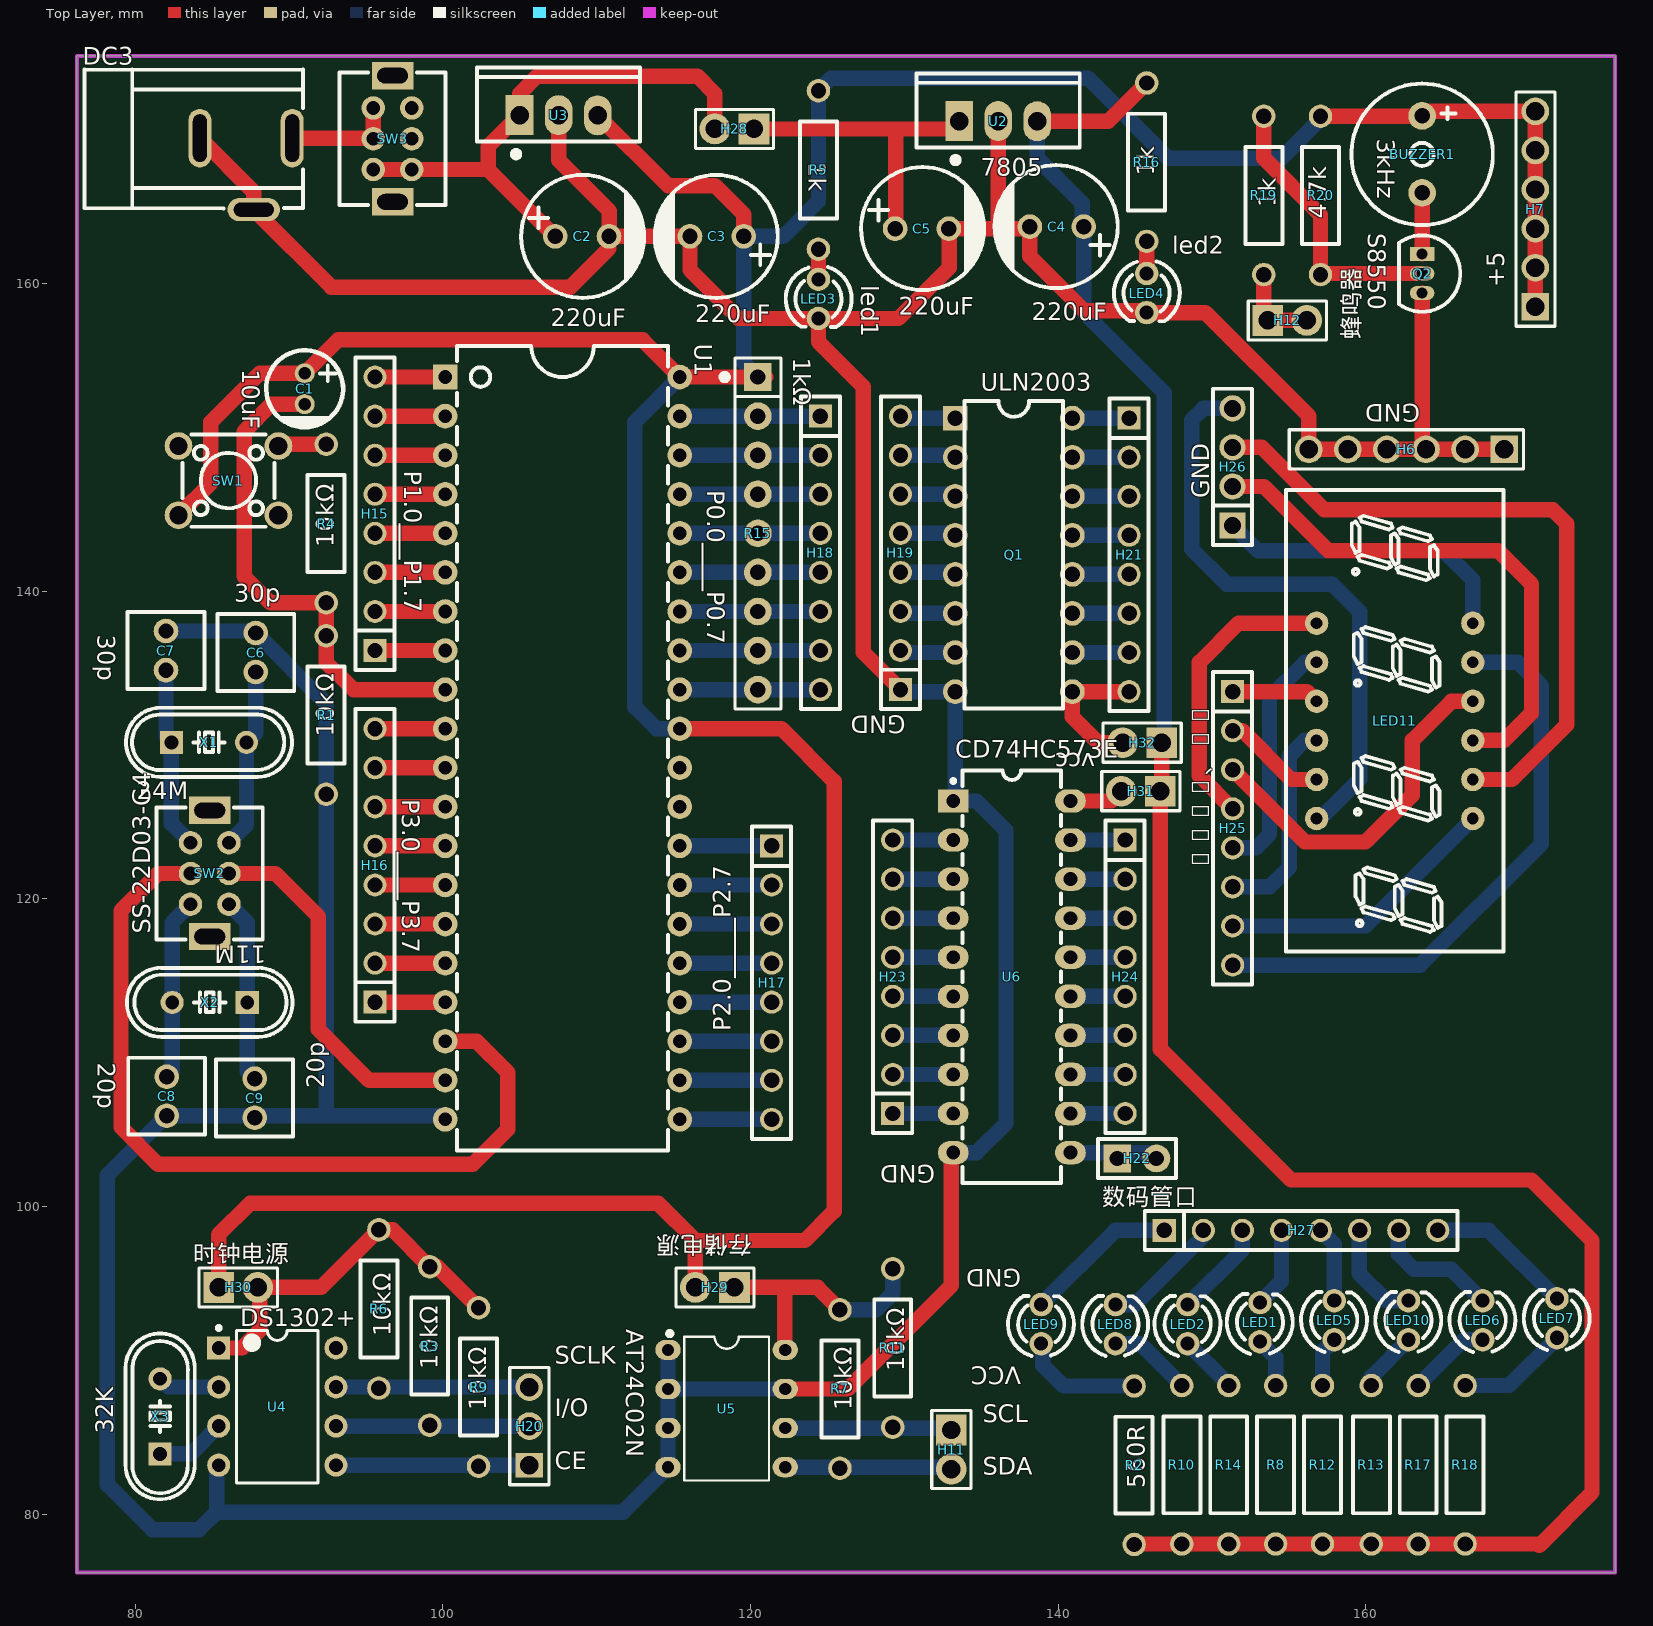
[diagram p0: Top Layer view]
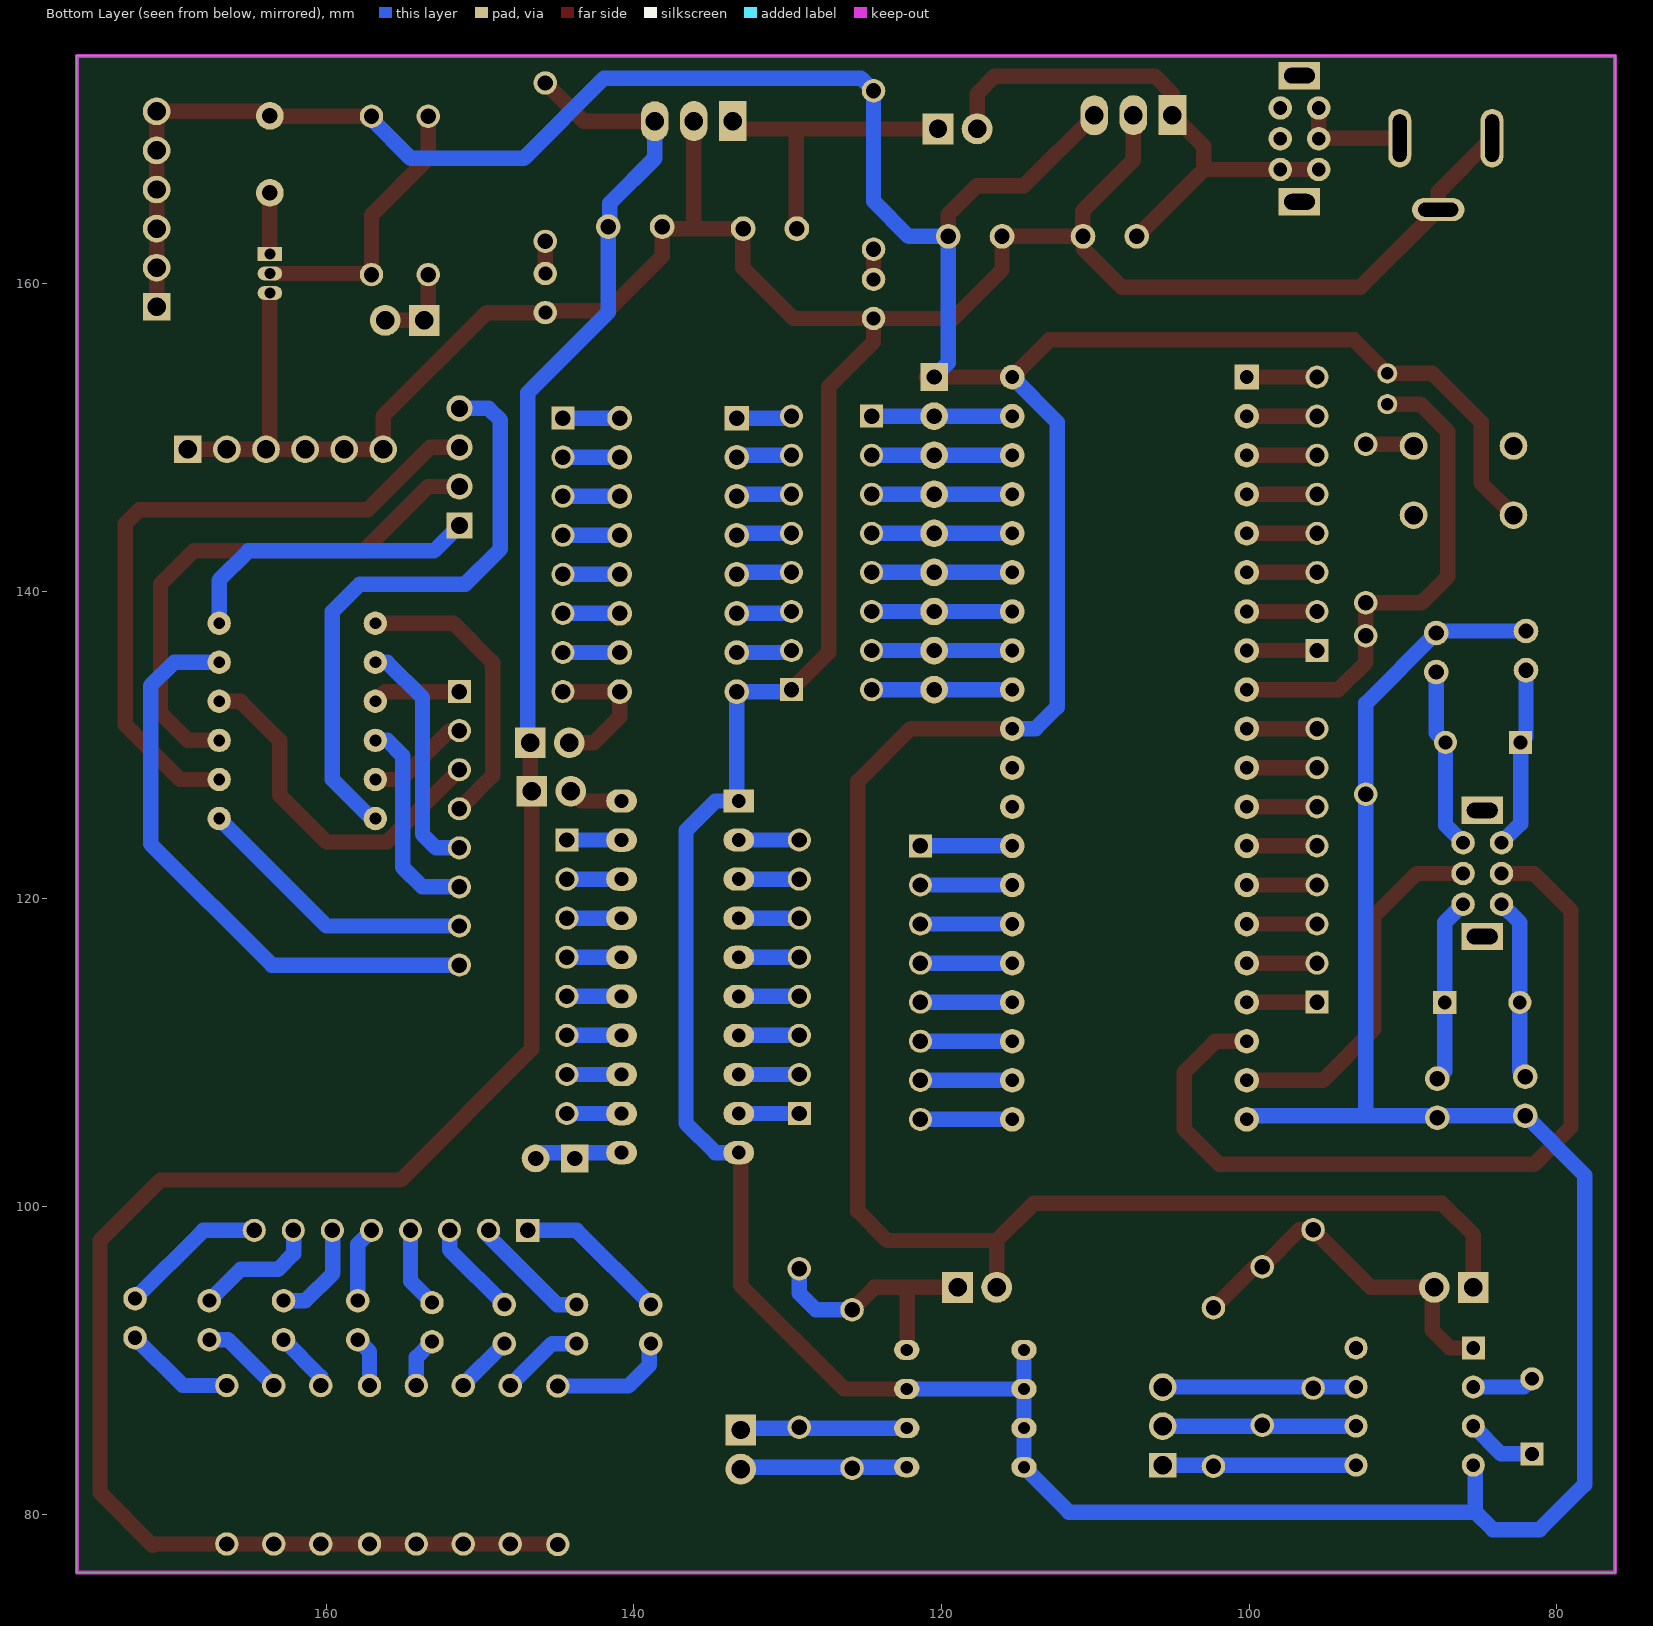
[diagram p1: Bottom Layer view, seen from below]
# Altium PCB MISC49922.pcbdoc
Units mm, origin at the board's own origin, x right, y up, seen from the top; angles counter-clockwise.
Board outline 100 x 98.6 mm, 2 copper layers (Top Layer, Bottom Layer), stack 1.58 mm thick; 78 components, 121 nets, 344 pads, 0 vias.

## Layer stack, top to bottom
Top Solder Mask Layer: solder mask 0.01, Dk 3.3
Top Layer: signal copper 0.035
Dielectric1: surface 1.51, FR4, Dk 4.5
Bottom Layer: signal copper 0.035
Bottom Solder Mask Layer: solder mask 0.01, Dk 3.3

## Board outline
76.2,174.803 76.2,76.2 176.2,76.2 176.2,174.803

## Design rules (kind name [scope] priority, off if disabled: settings)
BoardOutlineClearance copperThickness2oz_1 [All] p2 off: genericclearance=0.203 ignorepadtopadclearanceinfootprint=FALSE except(0: Arc-SplitContinuation Track-SplitContinuation SMDPad-SplitContinuation THPad-SplitContinuation Via-SplitContinuation Fill-SplitContinuation Region-SplitContinuation Poly-SplitContinuation Text-SplitContinuation Hole-SplitContinuation; 0.152: SMDPad-CutoutEdge THPad-CutoutEdge Via-CutoutEdge Fill-CutoutEdge Region-CutoutEdge Text-CutoutEdge Hole-CutoutEdge; 0.254: Poly-OutlineEdge Poly-CutoutEdge; 0.3: Arc-OutlineEdge Track-OutlineEdge SMDPad-OutlineEdge THPad-OutlineEdge Via-OutlineEdge Fill-OutlineEdge Region-OutlineEdge Text-OutlineEdge Hole-OutlineEdge Arc-CutoutEdge Track-CutoutEdge)
BoardOutlineClearance Plane_innerPlane_1 [All] p4 off: genericclearance=0.102 ignorepadtopadclearanceinfootprint=FALSE except(0: Arc-SplitContinuation Track-SplitContinuation SMDPad-SplitContinuation THPad-SplitContinuation Via-SplitContinuation Fill-SplitContinuation Region-SplitContinuation Poly-SplitContinuation Text-SplitContinuation Hole-SplitContinuation; 0.152: SMDPad-CutoutEdge THPad-CutoutEdge Via-CutoutEdge Fill-CutoutEdge Region-CutoutEdge Text-CutoutEdge Hole-CutoutEdge; 0.254: Poly-OutlineEdge Poly-CutoutEdge; 0.3: Arc-OutlineEdge Track-OutlineEdge SMDPad-OutlineEdge THPad-OutlineEdge Via-OutlineEdge Fill-OutlineEdge Region-OutlineEdge Text-OutlineEdge Hole-OutlineEdge Arc-CutoutEdge Track-CutoutEdge)
BoardOutlineClearance Copper_copperRegion_1 [All] p6 off: genericclearance=0.102 ignorepadtopadclearanceinfootprint=FALSE except(0: Arc-SplitContinuation Track-SplitContinuation SMDPad-SplitContinuation THPad-SplitContinuation Via-SplitContinuation Fill-SplitContinuation Region-SplitContinuation Poly-SplitContinuation Text-SplitContinuation Hole-SplitContinuation; 0.152: SMDPad-CutoutEdge THPad-CutoutEdge Via-CutoutEdge Fill-CutoutEdge Region-CutoutEdge Text-CutoutEdge Hole-CutoutEdge; 0.254: Poly-OutlineEdge Poly-CutoutEdge; 0.3: Arc-OutlineEdge Track-OutlineEdge SMDPad-OutlineEdge THPad-OutlineEdge Via-OutlineEdge Fill-OutlineEdge Region-OutlineEdge Text-OutlineEdge Hole-OutlineEdge Arc-CutoutEdge Track-CutoutEdge)
BoardOutlineClearance copperThickness1oz_1 [All] p8: genericclearance=0.102 ignorepadtopadclearanceinfootprint=FALSE except(0: Arc-SplitContinuation Track-SplitContinuation SMDPad-SplitContinuation THPad-SplitContinuation Via-SplitContinuation Fill-SplitContinuation Region-SplitContinuation Poly-SplitContinuation Text-SplitContinuation Hole-SplitContinuation; 0.152: SMDPad-CutoutEdge THPad-CutoutEdge Via-CutoutEdge Fill-CutoutEdge Region-CutoutEdge Text-CutoutEdge Hole-CutoutEdge; 0.254: Poly-OutlineEdge Poly-CutoutEdge; 0.3: Arc-OutlineEdge Track-OutlineEdge SMDPad-OutlineEdge THPad-OutlineEdge Via-OutlineEdge Fill-OutlineEdge Region-OutlineEdge Text-OutlineEdge Hole-OutlineEdge Arc-CutoutEdge Track-CutoutEdge)
Clearance copperThickness2oz [All] p1 off: gap=0.203 ignorepadtopadclearanceinfootprint=FALSE except(0.152: SMDPad-Track SMDPad-SMDPad THPad-Track SMDPad-THPad THPad-THPad Track-Via SMDPad-Via THPad-Via Via-Via Fill-Track Region-Track Fill-SMDPad Region-SMDPad Fill-THPad Region-THPad Fill-Via Region-Via Fill-Fill Fill-Region Region-Region Arc-Track Arc-SMDPad Arc-THPad Arc-Via Fill-Arc Region-Arc Arc-Arc Text-Track SMDPad-Text Text-THPad Text-Via Fill-Text Region-Text Arc-Text Text-Text Hole-Track Hole-SMDPad Hole-THPad Hole-Via Fill-Hole Region-Hole Hole-Arc Hole-Text; 0.254: Poly-Track Poly-SMDPad Poly-THPad Poly-Via Poly-Fill Poly-Region Poly-Poly Poly-Arc Poly-Text Poly-Hole)
Clearance Plane_innerPlane [All] p3 off: gap=0.102 ignorepadtopadclearanceinfootprint=FALSE except(0.152: SMDPad-Track SMDPad-SMDPad THPad-Track SMDPad-THPad THPad-THPad Track-Via SMDPad-Via THPad-Via Via-Via Fill-Track Region-Track Fill-SMDPad Region-SMDPad Fill-THPad Region-THPad Fill-Via Region-Via Fill-Fill Fill-Region Region-Region Arc-Track Arc-SMDPad Arc-THPad Arc-Via Fill-Arc Region-Arc Arc-Arc Text-Track SMDPad-Text Text-THPad Text-Via Fill-Text Region-Text Arc-Text Text-Text Hole-Track Hole-SMDPad Hole-THPad Hole-Via Fill-Hole Region-Hole Hole-Arc Hole-Text; 0.254: Poly-Track Poly-SMDPad Poly-THPad Poly-Via Poly-Fill Poly-Region Poly-Poly Poly-Arc Poly-Text Poly-Hole)
Clearance Copper_copperRegion [All] p5 off: gap=0.102 ignorepadtopadclearanceinfootprint=FALSE except(0.152: SMDPad-Track SMDPad-SMDPad THPad-Track SMDPad-THPad THPad-THPad Track-Via SMDPad-Via THPad-Via Via-Via Fill-Track Region-Track Fill-SMDPad Region-SMDPad Fill-THPad Region-THPad Fill-Via Region-Via Fill-Fill Fill-Region Region-Region Arc-Track Arc-SMDPad Arc-THPad Arc-Via Fill-Arc Region-Arc Arc-Arc Text-Track SMDPad-Text Text-THPad Text-Via Fill-Text Region-Text Arc-Text Text-Text Hole-Track Hole-SMDPad Hole-THPad Hole-Via Fill-Hole Region-Hole Hole-Arc Hole-Text; 0.254: Poly-Track Poly-SMDPad Poly-THPad Poly-Via Poly-Fill Poly-Region Poly-Poly Poly-Arc Poly-Text Poly-Hole)
Clearance copperThickness1oz [All] p7: gap=0.102 ignorepadtopadclearanceinfootprint=FALSE except(0.152: SMDPad-Track SMDPad-SMDPad THPad-Track SMDPad-THPad THPad-THPad Track-Via SMDPad-Via THPad-Via Via-Via Fill-Track Region-Track Fill-SMDPad Region-SMDPad Fill-THPad Region-THPad Fill-Via Region-Via Fill-Fill Fill-Region Region-Region Arc-Track Arc-SMDPad Arc-THPad Arc-Via Fill-Arc Region-Arc Arc-Arc Text-Track SMDPad-Text Text-THPad Text-Via Fill-Text Region-Text Arc-Text Text-Text Hole-Track Hole-SMDPad Hole-THPad Hole-Via Fill-Hole Region-Hole Hole-Arc Hole-Text; 0.254: Poly-Track Poly-SMDPad Poly-THPad Poly-Via Poly-Fill Poly-Region Poly-Poly Poly-Arc Poly-Text Poly-Hole)
DiffPairsRouting differentialPair [All] p1: maxlimit=0.152 minlimit=0.152 mostfreqgap=0.152 toplayer_minwidth=0.127 toplayer_prefwidth=0.254 toplayer_maxwidth=2.54 toplayer_mingap=0.152 toplayer_prefgap=0.152 toplayer_maxgap=0.152 bottomlayer_minwidth=0.127 bottomlayer_prefwidth=0.254 bottomlayer_maxwidth=2.54 bottomlayer_mingap=0.152 bottomlayer_prefgap=0.152 bottomlayer_maxgap=0.152 maxuncoupledlength=0.254
HoleToHoleClearance otherClearance [All] p1: gap=0.3 allowstackedmicrovias=TRUE
Length netLength [All] p1: minlimit=0 maxlimit=0
PasteMaskExpansion pasteMaskExpansion [All] p1: expansion=0
PlaneConnect innerPlane [All] p1: planeconnectstyle=Relief reliefexpansion=0.508 reliefentries=4 reliefconductorwidth=0.254 reliefairgap=0.254
PolygonConnect copperRegion [All] p1: connectstyle=Relief reliefconductorwidth=0.254 reliefentries=4 polygonreliefangle="90 Angle" airgapwidth=0.254 via.connectstyle=Relief via.reliefconductorwidth=0.254 via.reliefentries=4 via.polygonreliefangle="90 Angle" via.airgapwidth=0.254
RoutingVias viaSize [All] p1: holewidth=0.305 width=0.61 viastyle="Through Hole" minholewidth=0.3 minwidth=0.5 maxholewidth=6.3 maxwidth=10
SolderMaskExpansion solderMaskExpansion [IsVia] p1: expansion=-25.4 istentingtop=TRUE
SolderMaskExpansion solderMaskExpansion [All] p2: expansion=0.051 istentingtop=FALSE
Width copperThickness2oz_2 [All] p1 off: maxlimit=2.54 minlimit=0.203 preferedwidth=0.254
Width copperThickness1oz_2 [All] p2: maxlimit=2.54 minlimit=0.127 preferedwidth=0.254

## Components (designator, comment, footprint, x,y, rotation, side; value= is the part's Value field where it differs from the comment)
BUZZER1 "3kHz" BUZ-TH_BD9.0-P5.00-D0.6-FD 163.652,168.402 r270 top
C1 "10uF" CAP-TH_BD5.0-P2.00-D0.8-FD 91.008,153.162 r270 top
C2 "220uF" CAP-TH_BD8.0-P3.50-D0.6-FD 109.042,163.068 r0 top
C3 "220uF" CAP-TH_BD8.0-P3.50-D0.6-FD 117.805,163.068 r180 top
C4 "220uF" CAP-TH_BD8.0-P3.50-D0.6-FD 139.903,163.703 r180 top
C5 "220uF" CAP-TH_BD8.0-P3.50-D0.6-FD 131.14,163.576 r0 top
C6 "30p" CAP-TH_L5.0-W5.0-P2.54-D1.0 87.833,136.017 r270 top
C7 "30p" CAP-TH_L5.0-W5.0-P2.54-D1.0 81.991,136.144 r270 top
C8 "20p" CAP-TH_L5.0-W5.0-P2.54-D1.0 82.041,107.174 r270 top
C9 "20p" CAP-TH_L5.0-W5.0-P2.54-D1.0 87.756,107.047 r90 top
DC3 "DC-005-20A" DC-IN-TH_DC-005-20A 87.198,167.132 r0 top
H6 "GND" HDR-TH_6P-P2.54-V-M-1 162.636,149.225 r180 top
H7 "+5" HDR-TH_6P-P2.54-V-M-1 171.018,164.846 r90 top
H11 "SCL /  / SDA" HDR-TH_2P-P2.54-V-M 133.045,84.201 r270 top
H12 "蜂鸣器" HDR-TH_2P-P2.54-V-M 154.889,157.607 r0 top
H15 "P1.0___P1.7" HDR-TH_8P-P2.54-V-M 95.58,145.034 r90 top
H16 "P3.0____P3.7" HDR-TH_8P-P2.54-V-M 95.58,122.174 r90 top
H17 "P2.0_____P2.7" HDR-TH_8P-P2.54-V-M 121.361,114.554 r270 top
H18 "P0.0____P0.7" HDR-TH_8P-P2.54-V-M 124.536,142.494 r270 top
H19 "PZ254V-11-08P" HDR-TH_8P-P2.54-V-M 129.743,142.494 r90 top
H20 "SCLK /  / I/O /  / CE" HDR-TH_3P-P2.54-V-M-1 105.613,85.725 r90 top
H21 "PZ254V-11-08P" HDR-TH_8P-P2.54-V-M 144.602,142.367 r270 top
H22 "数码管口" HDR-TH_2P-P2.54-V-M-1 145.11,103.124 r0 top
H23 "PZ254V-11-08P" HDR-TH_8P-P2.54-V-M 129.235,114.935 r90 top
H24 "PZ254V-11-08P" HDR-TH_8P-P2.54-V-M 144.348,114.935 r270 top
H25 "g--a、Dp" HDR-TH_8P-P2.54-V-M 151.333,124.587 r270 top
H26 "GND" HDR-TH_4P-P2.54-V-M 151.333,148.082 r90 top
H27 "PZ254V-11-08P" HDR-TH_8P-P2.54-V-M 155.781,98.452 r0 top
H28 "PZ254V-11-02P" HDR-TH_2P-P2.54-V-M 118.948,170.053 r180 top
H29 "存储电源" HDR-TH_2P-P2.54-V-M 117.678,94.742 r180 top
H30 "时钟电源" HDR-TH_2P-P2.54-V-M 86.69,94.742 r0 top
H31 "PZ254V-11-02P" HDR-TH_2P-P2.54-V-M 145.364,127 r180 top
H32 "PZ254V-11-02P" HDR-TH_2P-P2.54-V-M 145.458,130.153 r180 top
LED1 "204-10SURD/S530-A3-L" LED-TH_BD3.0-P2.54-FD 153.114,92.483 r90 top
LED2 "204-10SURD/S530-A3-L" LED-TH_BD3.0-P2.54-FD 148.415,92.356 r90 top
LED3 "led1" LED-TH_BD3.0-P2.54-FD 124.409,159.004 r270 top
LED4 "led2" LED-TH_BD3.0-P2.54-FD 145.745,159.385 r270 top
LED5 "204-10SURD/S530-A3-L" LED-TH_BD3.0-P2.54-FD 157.94,92.61 r90 top
LED6 "204-10SURD/S530-A3-L" LED-TH_BD3.0-P2.54-FD 167.592,92.61 r90 top
LED7 "204-10SURD/S530-A3-L" LED-TH_BD3.0-P2.54-FD 172.418,92.737 r90 top
LED8 "204-10SURD/S530-A3-L" LED-TH_BD3.0-P2.54-FD 143.716,92.356 r90 top
LED9 "204-10SURD/S530-A3-L" LED-TH_BD3.0-P2.54-FD 138.89,92.356 r90 top
LED10 "204-10SURD/S530-A3-L" LED-TH_BD3.0-P2.54-FD 162.766,92.61 r90 top
LED11 "FJ3461AH" LED-SEG-TH_12P-L30.0-W14.0-P2.54-S10.16-BL 161.874,131.572 r270 top
Q1 "ULN2003" DIP-16_L19.8-W6.5-P2.54-LS7.6-BL 137.109,142.367 r270 top
Q2 "S8550" TO-92-3_L4.9-W3.7-P1.27-L 163.652,160.655 r270 top
R1 "10kΩ" RES-TH_BD2.4-L6.3-P10.30-D0.6 92.405,131.953 r90 top
R2 "560R" RES-TH_BD2.4-L6.3-P10.30-D0.6 144.93,83.182 r90 top
R3 "10kΩ" RES-TH_BD2.4-L6.3-P10.30-D0.6 99.136,90.932 r90 top
R4 "10kΩ" RES-TH_BD2.4-L6.3-P10.30-D0.6 92.405,144.399 r90 top
R5 "1k" RES-TH_BD2.4-L6.3-P10.30-D0.6 124.409,167.386 r270 top
R6 "10kΩ" RES-TH_BD2.4-L6.3-P10.30-D0.6 95.834,93.345 r90 top
R7 "10kΩ" RES-TH_BD2.4-L6.3-P10.30-D0.6 125.806,88.138 r90 top
R8 "560R" RES-TH_BD2.4-L6.3-P10.30-D0.6 154.13,83.212 r90 top
R9 "10kΩ" RES-TH_BD2.4-L6.3-P10.30-D0.6 102.311,88.265 r90 top
R10 "560R" RES-TH_BD2.4-L6.3-P10.30-D0.6 148.034,83.212 r90 top
R11 "10kΩ" RES-TH_BD2.4-L6.3-P10.30-D0.6 129.235,90.805 r90 top
R12 "560R" RES-TH_BD2.4-L6.3-P10.30-D0.6 157.178,83.212 r90 top
R13 "560R" RES-TH_BD2.4-L6.3-P10.30-D0.6 160.353,83.212 r90 top
R14 "560R" RES-TH_BD2.4-L6.3-P10.30-D0.6 151.082,83.212 r90 top
R15 "1kΩ" RES-ARRAY-TH_9P-L22.8-W3.00-P2.54 120.472,143.764 r270 top
R16 "1k" RES-TH_BD2.4-L6.3-P10.30-D0.6 145.745,167.894 r90 top
R17 "560R" RES-TH_BD2.4-L6.3-P10.30-D0.6 163.401,83.212 r90 top
R18 "560R" RES-TH_BD2.4-L6.3-P10.30-D0.6 166.449,83.212 r90 top
R19 "1k" RES-TH_BD2.4-L6.3-P10.30-D0.6 153.365,165.735 r90 top
R20 "4.7k" RES-TH_BD2.4-L6.3-P10.30-D0.6 157.048,165.735 r90 top
SW1 "TS-1095-A7B2-D1" SW-TH_4P-L6.0-W6.0-P4.50-LS6.5 86.055,147.193 r0 top
SW2 "SS-22D03-G4" SW-TH_SS-22D03-G4 84.835,121.652 r270 top
SW3 "SS-22D03-G4" SW-TH_SS-22D03-G4 96.723,169.418 r90 top
U1 "STC89C52RC-40I-PDIP40" DIP-40_L52.0-W13.7-P2.54-LS15.2-BL 107.772,129.794 r270 top
U2 "7805" TO-220-3_L10.0-W4.5-P2.54-L 136.093,170.561 r0 top
U3 "7805" TO-220-3_L10.0-W4.5-P2.54-L 107.518,170.942 r0 top
U4 "DS1302+" DIP-8_L9.8-W6.6-P2.54-LS7.6-BL 89.23,86.995 r270 top
U5 "AT24C02N" DIP-8_L9.2-W6.3-P2.54-LS7.62-BL 118.44,86.868 r270 top
U6 "CD74HC573E" DIP-20_L26.8-W6.4-P2.54-LS7.6-BL 136.982,114.935 r270 top
X1 "24M" HC-49US_L11.5-W4.5-P4.88 84.785,130.175 r0 top
X2 "11M" HC-49US_L11.5-W4.5-P4.88 84.835,113.27 r180 top
X3 "32K" HC-49US_L11.5-W4.5-P4.88 81.61,86.36 r90 top

## Footprints (in the part's own frame and the unit in brackets; to place one, negate y for a bottom-side part, rotate by r counter-clockwise, add the part's x,y. Pads: shape width x height; smd on the part's side, far side on the other; paste and mask are expansions set on the pad)
BUZ-TH_BD9.0-P5.00-D0.6-FD [mm]
  round 1.8 hole 1 copper offset 0,0 paste+0 mask+0.051: 1(-2.5,0)
  round 1.8 hole 1 paste+0 mask+0.051: 2(2.5,0)
  silkscreen extent -4.6,-4.6 4.6,4.6
CAP-TH_BD5.0-P2.00-D0.8-FD [mm]
  round 1.3 hole 0.8 paste+0 mask+0.051: 1(-1,0) 2(1,0)
  silkscreen extent -2.5,-2.5 2.5,2.5
CAP-TH_BD8.0-P3.50-D0.6-FD [mm]
  round 1.6 hole 1 paste+0 mask+0.051: 1(-1.75,0) 2(1.75,0)
  silkscreen extent -3.96,-4 4.04,4
CAP-TH_L5.0-W5.0-P2.54-D1.0 [mm]
  round 1.6 hole 1 paste+0 mask+0.051: 1(-1.27,0) 2(1.27,0)
  silkscreen extent -2.5,-2.5 2.5,2.5
DC-IN-TH_DC-005-20A [mm]
  oval 1.5x3.8 hole 0.9 slot 3.1 at 90 deg copper offset -0.001,0 paste+0 mask+0.051: 1(3.001,2.325)
  oval 1.5x3.8 hole 0.9 slot 3.1 at 90 deg copper offset 0,0 paste+0 mask+0.051: 2(-3.001,2.325)
  oval 3.4x1.5 hole 0.9 slot 2.6 at 0 deg copper offset -0.001,0 paste+0 mask+0.051: 3(0.501,-2.325)
  silkscreen extent -10.51,-2.24 3.71,6.78
DIP-8_L9.2-W6.3-P2.54-LS7.62-BL [mm]
  oval 1.32x1.65 hole 0.8 paste+0 mask+0.051: 1(-3.81,-3.81) 2(-1.27,-3.81) 3(1.27,-3.81) 4(3.81,-3.81) 5(3.81,3.81) 6(1.27,3.81) 7(-1.27,3.81) 8(-3.81,3.81)
  silkscreen extent -5.02,-3.85 4.68,2.76
DIP-8_L9.8-W6.6-P2.54-LS7.6-BL [mm]
  rect 1.5x1.5 hole 0.9 paste+0 mask+0.051: 1(-3.81,-3.81)
  round 1.5 hole 0.9 paste+0 mask+0.051: 2(-1.27,-3.81) 3(1.27,-3.81) 4(3.81,-3.81) 5(3.81,3.81) 6(1.27,3.81) 7(-1.27,3.81) 8(-3.81,3.81)
  silkscreen extent -5.23,-3.93 4.96,2.65
DIP-16_L19.8-W6.5-P2.54-LS7.6-BL [mm]
  rect 1.6x1.6 hole 1 paste+0 mask+0.051: 1(-8.89,-3.81)
  round 1.6 hole 1 copper offset 0,0 paste+0 mask+0.051: 2(-6.35,-3.81) 3(-3.81,-3.81) 4(-1.27,-3.81) 5(1.27,-3.81) 6(3.81,-3.81) 7(6.35,-3.81) 8(8.89,-3.81) 9(8.89,3.81) 10(6.35,3.81) 11(3.81,3.81) 12(1.27,3.81) 13(-1.27,3.81) 14(-3.81,3.81) 15(-6.35,3.81) 16(-8.89,3.81)
  silkscreen extent -10,-3.2 10,3.2
DIP-20_L26.8-W6.4-P2.54-LS7.6-BL [mm]
  rect 1.5x2 hole 0.9 paste+0 mask+0.051: 1(-11.43,-3.81)
  oval 1.5x2 hole 0.9 paste+0 mask+0.051: 2(-8.89,-3.81) 3(-6.35,-3.81) 4(-3.81,-3.81) 5(-1.27,-3.81) 6(1.27,-3.81) 7(3.81,-3.81) 8(6.35,-3.81) 9(8.89,-3.81)
  oval 1.524x2 hole 0.9 paste+0 mask+0.051: 10(11.43,-3.81) 11(11.43,3.81) 12(8.89,3.81) 13(6.35,3.81) 14(3.81,3.81) 15(1.27,3.81) 16(-1.27,3.81) 17(-3.81,3.81) 18(-6.35,3.81) 19(-8.89,3.81) 20(-11.43,3.81)
  silkscreen extent -13.4,-3.93 13.4,3.2
DIP-40_L52.0-W13.7-P2.54-LS15.2-BL [mil]
  rect 63x63 hole 35 paste+0 mask+2: 1(-950,-300)
  round 63 hole 35 paste+0 mask+2: 2(-850,-300) 3(-750,-300) 4(-650,-300) 5(-550,-300) 6(-450,-300) 7(-350,-300) 8(-250,-300) 9(-150,-300) 10(-50,-300) 11(50,-300) 12(150,-300) 13(250,-300) 14(350,-300) 15(450,-300) 16(550,-300) 17(650,-300) 18(750,-300) 19(850,-300) 20(950,-300) 21(950,300) 22(850,300) 23(750,300) 24(650,300) 25(550,300) 26(450,300) 27(350,300) 28(250,300) 29(150,300) 30(50,300) 31(-50,300) 32(-150,300) 33(-250,300) 34(-350,300) 35(-450,300) 36(-550,300) 37(-650,300) 38(-750,300) 39(-850,300) 40(-950,300)
  silkscreen extent -1030,-270 1030,270
HC-49US_L11.5-W4.5-P4.88 [mm]
  rect 1.5x1.5 hole 0.9 paste+0 mask+0.051: 1(-2.44,0)
  round 1.5 hole 0.9 paste+0 mask+0.051: 2(2.44,0)
  silkscreen extent -5.39,-2.25 5.39,2.25
HDR-TH_2P-P2.54-V-M [mm]
  rect 2x2 hole 1.2 paste+0 mask+0.051: 1(-1.27,0)
  round 2 hole 1.2 paste+0 mask+0.051: 2(1.27,0)
  silkscreen extent -2.54,-1.27 2.54,1.27
HDR-TH_2P-P2.54-V-M-1 [mm]
  rect 1.8x1.8 hole 1 paste+0 mask+0.051: 1(-1.27,0)
  round 1.8 hole 1 paste+0 mask+0.051: 2(1.27,0)
  silkscreen extent -2.54,-1.27 2.54,1.27
HDR-TH_3P-P2.54-V-M-1 [mm]
  rect 1.575x1.8 hole 1.2 paste+0 mask+0.051: 1(-2.54,0)
  round 1.8 hole 1.2 paste+0 mask+0.051: 2(0,0) 3(2.54,0)
  silkscreen extent -3.81,-1.27 3.81,1.27
HDR-TH_4P-P2.54-V-M [mm]
  rect 1.7x1.7 hole 1.1 paste+0 mask+0.051: 1(-3.81,0)
  round 1.7 hole 1.1 paste+0 mask+0.051: 2(-1.27,0) 3(1.27,0) 4(3.81,0)
  silkscreen extent -5.08,-1.27 5.08,1.27
HDR-TH_6P-P2.54-V-M-1 [mm]
  rect 1.8x1.8 hole 1.2 paste+0 mask+0.051: 1(-6.35,0)
  round 1.8 hole 1.2 paste+0 mask+0.051: 2(-3.81,0) 3(-1.27,0) 4(1.27,0) 5(3.81,0) 6(6.35,0)
  silkscreen extent -7.62,-1.27 7.62,1.27
HDR-TH_8P-P2.54-V-M [mm]
  rect 1.5x1.5 hole 1 paste+0 mask+0.051: 1(-8.89,0)
  round 1.5 hole 1 paste+0 mask+0.051: 2(-6.35,0) 3(-3.81,0) 4(-1.27,0) 5(1.27,0) 6(3.81,0) 7(6.35,0) 8(8.89,0)
  silkscreen extent -10.16,-1.27 10.16,1.27
LED-SEG-TH_12P-L30.0-W14.0-P2.54-S10.16-BL [mil]
  round 60 hole 30 paste+0 mask+2: 1(-250,-200) 2(-150,-200) 3(-50,-200) 4(50,-200) 5(150,-200) 6(250,-200) 7(250,200) 8(150,200) 9(50,200) 10(-50,200) 11(-150,200) 12(-250,200)
  silkscreen extent -591,-279 591,279
LED-TH_BD3.0-P2.54-FD [mil]
  round 60 hole 36 paste+0 mask+2: 1(-50,0) 2(50,0)
  silkscreen extent -81,-84 72,85
RES-ARRAY-TH_9P-L22.8-W3.00-P2.54 [mm]
  rect 1.8x1.8 hole 1 paste+0 mask+0.051: 1(-10.16,0)
  round 1.8 hole 1 paste+0 mask+0.051: 2(-7.62,0) 3(-5.08,0) 4(-2.54,0) 5(0,0) 6(2.54,0) 7(5.08,0) 8(7.62,0) 9(10.16,0)
  silkscreen extent -11.41,-2.36 11.41,1.5
RES-TH_BD2.4-L6.3-P10.30-D0.6 [mm]
  round 1.524 hole 1 paste+0 mask+0.051: 1(-5.15,0) 2(5.15,0)
  silkscreen extent -3.15,-1.2 3.15,1.2
SW-TH_4P-L6.0-W6.0-P4.50-LS6.5 [mm]
  round 1.8 hole 1.2 paste+0 mask+0.051: 1(-3.25,2.25) 2(3.25,2.25) 3(-3.25,-2.25) 4(3.25,-2.25)
  silkscreen extent -3,-3 3,3
SW-TH_SS-22D03-G4 [mil]
  round 60 hole 35 paste+0 mask+2: 1(-78.73,49.22) 2(0.01,49.22) 3(78.75,49.22) 4(-78.73,-49.21) 5(0.01,-49.21) 6(78.75,-49.21)
  rect 70x106.3 hole 40 slot 78.74 at 90 deg copper offset -0.01,0.01 paste+0 mask+2: 7(-161.41,0)
  rect 70x106.3 hole 40 slot 78.74 at 90 deg paste+0 mask+2: 8(161.42,0)
  silkscreen extent -169,-136 169,136
TO-92-3_L4.9-W3.7-P1.27-L [mm]
  rect 0.9x1.6 hole 0.7 paste+0 mask+0.051: 1(-1.27,0)
  oval 0.9x1.6 hole 0.7 paste+0 mask+0.051: 2(0,0) 3(1.27,0)
  silkscreen extent -2.48,-1.5 2.48,2.48
TO-220-3_L10.0-W4.5-P2.54-L [mm]
  rect 1.8x2.6 hole 1.2 paste+0 mask+0.051: 1(-2.54,0.005)
  oval 1.8x2.6 hole 1.2 paste+0 mask+0.051: 2(0,0.005)
  oval 1.8x2.6 hole 1.2 copper offset 0,0 paste+0 mask+0.051: 3(2.54,-0.005)
  silkscreen extent -5.3,-2.73 5.3,3.09

## Nets (pads, with @x,y where several pads share a name; then routed paths per layer and width w, separated by ;. In a path a pad name is that pad's centre, name@x,y a point inside that pad or via, vN(x,y) a via of type N, cw(c..) or ccw(c..) an arc to the next point about the centre after c; other vN are vias at no path point)
5C: H29.1 R7.2 R11.2 U5.8 | length 17
  Top Layer w1: H29.1 122.207,94.742 ; U5.8 122.207,90.721 122.207,94.742 ; R7.2 124.352,94.742 122.207,94.742
  Bottom Layer w1: R7.2 128.162,93.288 129.235,94.361 R11.2
5S: H30.2 R3.2 R6.2 R9.2 U4.1 | length 24
  Top Layer w1: U4.1 86.944,90.805 88.087,91.948 88.087,94.615 H30.2 92.081,94.742 R6.2 96.723,98.495 R3.2 99.644,96.082 R9.2
$1N4569: C6.2 SW2.1 X1.2 | length 11.8
  Bottom Layer w1: SW2.1 87.225,124.791 X1.2 87.833,130.783 C6.2
$1N4573: C7.2 SW2.4 X1.1 | length 11.9
  Bottom Layer w1: C7.2 81.991,130.529 X1.1 82.345,124.892 SW2.4
$1N4577: C9.2 SW2.3 X2.1 | length 12
  Bottom Layer w1: SW2.3 87.275,118.462 X2.1 87.275,108.798 C9.2
$1N4581: C8.1 SW2.6 X2.2 | length 11.8
  Bottom Layer w1: C8.1 82.395,108.798 X2.2 82.395,118.462 SW2.6
$1N4821: C1.2 R1.2 R4.1 U1.9 | length 32.5
  Top Layer w1: C1.2 88.865,152.162 87.071,150.368 87.071,140.97 88.792,139.249 R4.1 R1.2 92.405,135.382 94.183,133.604 U1.9
$1N4832: R4.2 SW1.2 | length 3.1
  Top Layer w1: SW1.2 89.411,149.549 R4.2
$1N4836: SW2.5 U1.18 | length 55.3
  Top Layer w1: SW2.5 81.483,121.652 79.07,119.239 79.07,105.156 81.483,102.743 101.93,102.743 104.216,105.029 104.216,108.712 102.184,110.744 U1.18
$1N4841: SW2.2 U1.19 | length 23.9
  Top Layer w1: SW2.2 89.103,121.652 91.897,118.858 91.897,111.506 95.199,108.204 U1.19
$1N4907: H15.1 U1.8 | length 4.6
  Top Layer w1: H15.1 U1.8
$1N4909: H15.2 U1.7 | length 4.6
  Top Layer w1: H15.2 U1.7
$1N4911: H15.3 U1.6 | length 4.6
  Top Layer w1: H15.3 U1.6
$1N4913: H15.4 U1.5 | length 4.6
  Top Layer w1: H15.4 U1.5
$1N4915: H15.5 U1.4 | length 4.6
  Top Layer w1: H15.5 U1.4
$1N4917: H15.6 U1.3 | length 4.6
  Top Layer w1: H15.6 U1.3
$1N4919: H15.7 U1.2 | length 4.6
  Top Layer w1: H15.7 U1.2
$1N4921: H15.8 U1.1 | length 4.6
  Top Layer w1: H15.8 U1.1
$1N4984: H16.1 U1.17 | length 4.6
  Top Layer w1: H16.1 U1.17
$1N4986: H16.2 U1.16 | length 4.6
  Top Layer w1: H16.2 U1.16
$1N4988: H16.3 U1.15 | length 4.6
  Top Layer w1: H16.3 U1.15
$1N4990: H16.4 U1.14 | length 4.6
  Top Layer w1: H16.4 U1.14
$1N4992: H16.5 U1.13 | length 4.6
  Top Layer w1: H16.5 U1.13
$1N4994: H16.6 U1.12 | length 4.6
  Top Layer w1: H16.6 U1.12
$1N4996: H16.7 U1.11 | length 4.6
  Top Layer w1: H16.7 U1.11
$1N4998: H16.8 U1.10 | length 4.6
  Top Layer w1: H16.8 U1.10
$1N5061: H17.1 U1.28 | length 6
  Bottom Layer w1: U1.28 H17.1
$1N5063: H17.2 U1.27 | length 6
  Bottom Layer w1: U1.27 H17.2
$1N5065: H17.3 U1.26 | length 6
  Bottom Layer w1: U1.26 H17.3
$1N5067: H17.4 U1.25 | length 6
  Bottom Layer w1: U1.25 H17.4
$1N5069: H17.5 U1.24 | length 6
  Bottom Layer w1: U1.24 H17.5
$1N5071: H17.6 U1.23 | length 6
  Bottom Layer w1: U1.23 H17.6
$1N5073: H17.7 U1.22 | length 6
  Bottom Layer w1: U1.22 H17.7
$1N5075: H17.8 U1.21 | length 6
  Bottom Layer w1: U1.21 H17.8
$1N5260: H18.1 R15.2 U1.39 | length 9.1
  Bottom Layer w1: U1.39 120.98,151.384 H18.1
$1N5262: H18.2 R15.3 U1.38 | length 9.1
  Bottom Layer w1: U1.38 120.98,148.844 H18.2
$1N5264: H18.3 R15.4 U1.37 | length 9.1
  Bottom Layer w1: U1.37 120.98,146.304 H18.3
$1N5266: H18.4 R15.5 U1.36 | length 9.1
  Bottom Layer w1: U1.36 120.98,143.764 H18.4
$1N5268: H18.5 R15.6 U1.35 | length 9.1
  Bottom Layer w1: U1.35 120.98,141.224 H18.5
$1N5270: H18.6 R15.7 U1.34 | length 9.1
  Bottom Layer w1: U1.34 120.98,138.684 H18.6
$1N5272: H18.7 R15.8 U1.33 | length 9.1
  Bottom Layer w1: U1.33 120.98,136.144 H18.7
$1N5274: H18.8 R15.9 U1.32 | length 9.1
  Bottom Layer w1: U1.32 120.98,133.604 H18.8
$1N5508: C5.1 H28.1 U2.1 | length 20
  Top Layer w1: H28.1 129.433,170.053 ; C5.1 129.433,163.619 129.433,170.053 ; U2.1 133.04,170.053 129.433,170.053
$1N5583: LED3.1 R5.2 | length 2
  Top Layer w1: LED3.1 R5.2
$1N5696: LED4.1 R16.1 | length 2.1
  Top Layer w1: LED4.1 R16.1
$1N5745: U4.2 X3.2 | length 4
  Bottom Layer w1: X3.2 82.145,88.265 U4.2
$1N5749: U4.3 X3.1 | length 4.6
  Bottom Layer w1: X3.1 83.615,83.92 U4.3
$1N5942: H20.3 R6.1 U4.7 | length 12.6
  Bottom Layer w1: U4.7 H20.3
$1N5945: H20.2 R3.1 U4.6 | length 12.6
  Bottom Layer w1: U4.6 H20.2
$1N5948: H20.1 R9.1 U4.5 | length 12.6
  Bottom Layer w1: U4.5 H20.1
$1N5955: H19.2 Q1.7 | length 3.6
  Bottom Layer w1: H19.2 129.87,136.017 Q1.7
$1N5957: H19.3 Q1.6 | length 3.6
  Bottom Layer w1: H19.3 129.87,138.557 Q1.6
$1N5959: H19.4 Q1.5 | length 3.6
  Bottom Layer w1: H19.4 133.172,141.224 Q1.5
$1N5961: H19.5 Q1.4 | length 3.6
  Bottom Layer w1: H19.5 133.172,143.764 Q1.4
$1N5963: H19.6 Q1.3 | length 3.6
  Bottom Layer w1: H19.6 133.172,146.304 Q1.3
$1N5965: H19.7 Q1.2 | length 3.6
  Bottom Layer w1: H19.7 133.172,148.844 Q1.2
$1N5967: H19.8 Q1.1 | length 3.6
  Bottom Layer w1: H19.8 129.87,151.257 Q1.1
$1N6030: H21.1 Q1.16 | length 3.7
  Bottom Layer w1: Q1.16 H21.1
$1N6032: H21.2 Q1.15 | length 3.7
  Bottom Layer w1: Q1.15 H21.2
$1N6034: H21.3 Q1.14 | length 3.7
  Bottom Layer w1: Q1.14 H21.3
$1N6036: H21.4 Q1.13 | length 3.7
  Bottom Layer w1: Q1.13 H21.4
$1N6038: H21.5 Q1.12 | length 3.7
  Bottom Layer w1: Q1.12 H21.5
$1N6040: H21.6 Q1.11 | length 3.7
  Bottom Layer w1: Q1.11 H21.6
$1N6042: H21.7 Q1.10 | length 3.7
  Bottom Layer w1: Q1.10 H21.7
$1N6203: H11.1 R11.1 U5.6 | length 10.8
  Bottom Layer w1: U5.6 132.918,85.598 H11.1
$1N6206: H11.2 R7.1 U5.5 | length 10.8
  Bottom Layer w1: U5.5 132.918,83.058 H11.2
$1N6330: H22.1 H22.2 U6.11 | length 5.7
  Bottom Layer w1: U6.11 145.999,103.505 H22.2
$1N6392: H23.1 U6.9 | length 3.9
  Bottom Layer w1: H23.1 U6.9
$1N6394: H23.2 U6.8 | length 3.9
  Bottom Layer w1: H23.2 U6.8
$1N6396: H23.3 U6.7 | length 3.9
  Bottom Layer w1: H23.3 U6.7
$1N6398: H23.4 U6.6 | length 3.9
  Bottom Layer w1: H23.4 U6.6
$1N6400: H23.5 U6.5 | length 3.9
  Bottom Layer w1: H23.5 U6.5
$1N6402: H23.6 U6.4 | length 3.9
  Bottom Layer w1: H23.6 U6.4
$1N6404: H23.7 U6.3 | length 3.9
  Bottom Layer w1: H23.7 U6.3
$1N6406: H23.8 U6.2 | length 3.9
  Bottom Layer w1: H23.8 U6.2
$1N6469: H24.1 U6.19 | length 3.6
  Bottom Layer w1: U6.19 H24.1
$1N6471: H24.2 U6.18 | length 3.6
  Bottom Layer w1: U6.18 H24.2
$1N6473: H24.3 U6.17 | length 3.6
  Bottom Layer w1: U6.17 H24.3
$1N6475: H24.4 U6.16 | length 3.6
  Bottom Layer w1: U6.16 H24.4
$1N6477: H24.5 U6.15 | length 3.6
  Bottom Layer w1: U6.15 H24.5
$1N6479: H24.6 U6.14 | length 3.6
  Bottom Layer w1: U6.14 H24.6
$1N6481: H24.7 U6.13 | length 3.6
  Bottom Layer w1: U6.13 H24.7
$1N6483: H24.8 U6.12 | length 3.6
  Bottom Layer w1: U6.12 H24.8
$1N6731: LED9.1 R2.2 | length 7.9
  Bottom Layer w1: LED9.1 138.99,90.986 138.99,89.692 140.35,88.332 R2.2
$1N6734: LED8.1 R10.2 | length 5.4
  Bottom Layer w1: LED8.1 145.31,91.086 R10.2
$1N6736: LED2.1 R14.2 | length 3.8
  Bottom Layer w1: LED2.1 151.082,88.419 R14.2
$1N6738: LED1.1 R8.2 | length 3.3
  Bottom Layer w1: LED1.1 154.13,90.197 R8.2
$1N6740: LED5.1 R12.2 | length 3.3
  Bottom Layer w1: R12.2 157.178,90.578 LED5.1
$1N6742: LED10.1 R13.2 | length 4
  Bottom Layer w1: R13.2 160.353,88.927 LED10.1
$1N6778: LED6.1 R17.2 | length 5.4
  Bottom Layer w1: R17.2 166.379,91.34 LED6.1
$1N6814: LED7.1 R18.2 | length 7.3
  Bottom Layer w1: R18.2 169.313,88.362 LED7.1
$1N6901: H27.1 LED9.2 | length 10
  Bottom Layer w1: LED9.2 143.716,98.452 H27.1
$1N6905: H27.8 LED7.2 | length 9.6
  Bottom Layer w1: H27.8 167.973,98.452 LED7.2
$1N6909: H27.7 LED6.2 | length 8.3
  Bottom Layer w1: H27.7 162.104,98.425 162.104,96.931 163.12,95.915 165.557,95.915 LED6.2
$1N6914: H27.6 LED10.2 | length 6.7
  Bottom Layer w1: H27.6 159.564,98.425 159.564,95.661 161.345,93.88 LED10.2
$1N6919: H27.5 LED5.2 | length 4.9
  Bottom Layer w1: H27.5 157.94,97.563 LED5.2
$1N6924: H27.4 LED1.2 | length 5.3
  Bottom Layer w1: LED1.2 154.511,95.15 H27.4
$1N6933: H27.2 LED8.2 | length 7.9
  Bottom Layer w1: LED8.2 144.986,93.626 149.431,98.071 H27.2
$1N6938: H27.3 LED2.2 | length 6.3
  Bottom Layer w1: LED2.2 151.971,97.182 H27.3
$1N6987: BUZZER1.2 Q2.1 | length 4
  Top Layer w1: Q2.1 BUZZER1.2
$1N7023: Q2.2 R19.2 R20.1 | length 18.3
  Top Layer w1: R19.2 153.365,168.148 157.048,164.465 R20.1 157.118,160.655 Q2.2@163.538,160.655
$1N7088: H12.1 H12.2 R19.1 | length 5.6
  Top Layer w1: R19.1 153.365,157.861 H12.1 H12.2
$1N10306: H25.8 LED11.11 | length 38.7
  Bottom Layer w1: H25.8 163.525,115.697 171.399,123.571 171.399,133.858 169.875,135.382 LED11.11
$1N10312: H25.7 LED11.7 | length 18.5
  Bottom Layer w1: H25.7 159.969,118.237 LED11.7
$1N10325: H25.6 LED11.4 | length 13.7
  Bottom Layer w1: H25.6 153.746,120.777 155.016,122.047 155.016,129.302 156.016,130.302 LED11.4
$1N10330: H25.5 LED11.2 | length 15.7
  Bottom Layer w1: H25.5 152.857,123.317 153.73,124.19 153.73,133.08 156.032,135.382 LED11.2
$1N10335: H25.4 LED11.1 | length 19.1
  Top Layer w1: H25.4 149.174,128.016 149.174,135.382 151.714,137.922 LED11.1
$1N10344: H25.3 LED11.10 | length 23.4
  Top Layer w1: H25.3 156.032,123.698 159.969,123.698 163.017,126.746 163.017,130.302 165.557,132.842 LED11.10
$1N10351: H25.2 LED11.5 | length 6.8
  Top Layer w1: H25.2 151.968,130.937 155.143,127.762 LED11.5
$1N10354: H25.1 LED11.3 | length 5.7
  Top Layer w1: H25.1 156.159,133.477 LED11.3
$1N10359: H26.1 LED11.12 | length 19.9
  Bottom Layer w1: H26.1 152.984,142.621 165.049,142.621 166.954,140.716 LED11.12
$1N10363: H26.2 LED11.9 | length 35
  Top Layer w1: H26.2 153.365,146.812 157.556,142.621 168.605,142.621 170.764,140.462 170.764,132.08 168.986,130.302 LED11.9
$1N10368: H26.3 LED11.8 | length 44.4
  Top Layer w1: H26.3 153.238,149.352 157.302,145.288 172.161,145.288 173.05,144.399 173.05,131.318 169.494,127.762 LED11.8
$1N10373: H26.4 LED11.6 | length 38.7
  Bottom Layer w1: H26.4 149.428,151.892 148.666,151.13 148.666,142.748 150.952,140.462 157.81,140.462 159.588,138.684 159.588,127.762 157.048,125.222 LED11.6
$1N15122: H31.2 U6.20 | length 3.6
  Top Layer w1: U6.20 143.459,126.365 H31.2
$1N15173: H21.8 H32.2 Q1.9 | length 9.3
  Top Layer w1: H32.2 142.592,130.153 140.919,131.826 Q1.9 H21.8
$1N17499: C2.1 H28.2 SW3.1 SW3.4 U3.1 | length 35.3
  Top Layer w1: SW3.1 SW3.4 102.942,167.418 ; C2.1 102.942,167.418 ; H28.2 117.678,172.339 116.535,173.482 106.121,173.482 104.978,172.339 U3.1 102.942,168.911 102.942,167.418
+5V: BUZZER1.1 C1.1 C3.1 H7.1 H7.2 H7.3 H7.4 H7.5 H7.6 H29.2 H30.1 R5.1 R15.1 R20.2 SW1.3 U1.31 U1.40 U3.3 | length 260.2
  Top Layer w1: SW1.3 84.912,147.05 84.912,151.003 88.071,154.162 C1.1 93.183,156.337 112.979,156.337 U1.40 R15.1@120.98,153.924 ; H30.1 85.42,98.171 87.452,100.203 113.995,100.203 116.408,97.79 ; U3.3 114.625,166.37 117.678,166.37 119.555,164.493 C3.1 ; U1.31 121.996,131.064 125.425,127.635 125.425,99.695 123.52,97.79 116.408,97.79 ; H29.2 116.408,97.79 ; R20.2 163.635,170.885 BUZZER1.1 163.946,171.196 H7.6 H7.5 H7.4 H7.3 H7.2 H7.1
  Bottom Layer w1: U1.31 113.868,131.064 112.471,132.461 112.471,151.003 U1.40 ; R15.1 119.555,154.841 C3.1 122.123,163.068 124.409,165.354 R5.1 125.228,173.355 141.935,173.355 147.142,168.148 154.508,168.148 157.048,170.688 R20.2
GND: C2.2 C3.2 C4.2 C5.2 C6.1 C7.1 C8.2 C9.1 DC3.2 DC3.3 H6.1 H6.2 H6.3 H6.4 H6.5 H6.6 H19.1 LED3.2 LED4.2 Q1.8 Q2.3 R1.1 U1.20 U2.2 U3.2 U4.4 U5.1 U5.2 U5.3 U5.4 U5.7 U6.1 U6.10 | length 361.3
  Top Layer w1: DC3.2 87.698,165.957 DC3.3 92.739,159.766 108.28,159.766 110.792,162.278 C2.2 ; U3.2 107.518,168.021 110.82,164.719 110.82,163.096 C2.2 ; U5.7 126.314,88.138 133.045,94.869 133.045,103.378 U6.10 ; H19.1 127.33,136.017 127.33,153.289 124.409,156.21 LED3.2 ; U2.2 136.093,163.652 136.168,163.576 ; Q2.3 163.652,149.479 H6.3 ; H6.1 H6.2 H6.3 ; C2.2 C3.2 116.055,160.881 119.202,157.734 LED3.2 ; LED3.2 129.616,157.734 132.918,161.036 132.918,163.548 C5.2 136.168,163.576 ; 136.168,163.576 138.026,163.576 C4.2 138.153,161.77 141.681,158.242 145.618,158.242 LED4.2 149.555,158.115 156.286,151.384 H6.6 H6.5 H6.4 H6.3
  Bottom Layer w1: C7.1 87.706,137.414 C6.1 92.405,132.715 R1.1 92.405,106.064 92.245,105.904 ; U4.4 85.293,83.058 85.293,80.137 ; U1.20 99.912,105.904 92.245,105.904 ; U5.1 U5.2 ; U5.7 U5.2 ; H19.1 129.87,133.477 Q1.8 133.299,126.492 U6.1 134.696,126.365 136.601,124.46 136.601,105.41 134.696,103.505 U6.10 ; 85.293,80.137 84.15,78.994 81.102,78.994 78.181,81.915 78.181,102.044 C8.2 92.245,105.904 ; 85.293,80.137 111.709,80.137 U5.4 U5.3 U5.2
VCC: DC3.1 SW3.2 SW3.3 | length 7.3
  Top Layer w1: DC3.1 SW3.2@95.434,169.457 ; SW3.2 SW3.2@95.434,169.457 ; SW3.3 95.473,169.496 SW3.2@95.434,169.457
VCC+: C4.1 H31.1 H32.1 R2.1 R8.1 R10.1 R12.1 R13.1 R14.1 R16.2 R17.1 R18.1 U2.3 | length 152.8
  Top Layer w1: U2.3 143.257,170.556 R16.2 ; R2.1 144.961,78.062 R10.1 R14.1 R8.1 R12.1 R13.1 R17.1 R18.1 171.188,78.062 171.272,77.978 174.701,81.407 174.701,97.79 170.764,101.727 155.143,101.727 146.634,110.236 H31.1 146.728,127.094 H32.1
  Bottom Layer w1: U2.3 138.633,168.148 141.554,165.227 141.554,163.802 C4.1 141.653,158.143 146.888,152.908 146.888,130.314 H32.1
pads on no net: SW1.1 SW1.4 SW2.7 SW2.8 SW3.5 SW3.6 SW3.7 SW3.8 U1.29 U1.30 U4.8

## Keep-outs
Board Outline Layer:
  the board outline again, w0.254

## Silkscreen, mask and mechanical layers (free items; w line width, h text height)
Top Silkscreen Layer:
  text "GND" at 130.092,131.918 h1.14 r180
  text "vcc" at 142.403,129.455 h1.14 r180
  text "GND" at 131.997,102.679 h1.14 r180
  text "GND" at 137.588,95.938 h1.14 r180
  text "VCC" at 137.585,89.599 h1.14 r180